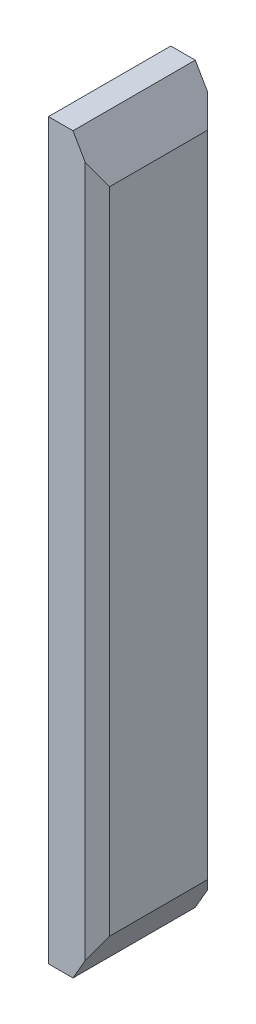
SolidWorks part; units mm, degrees
ref_plane "前视基准面" through (0, 0, 0) normal (0, 0, 1) x (1, 0, 0)
ref_plane "上视基准面" through (0, 0, 0) normal (0, 1, 0) x (1, 0, 0)
ref_plane "右视基准面" through (0, 0, 0) normal (1, 0, 0) x (0, 0, -1)
sketch "草图1" plane through (0, 0, 0) normal (1, 0, 0) x (0, 0, -1)
  line L1 (5, -30) -> (-5, -30)
  line L2 (5, -30) -> (5, 30)
  line L3 (5, 30) -> (-5, 30)
  line L4 (-5, -30) -> (-5, 30)
  line L5 (5, -30) -> (-5, 30) construction
  line L6 (5, 30) -> (-5, -30) construction
  point P0 (0, 0)
  dimension "D1" = 10
  dimension "D2" = 60
extrude "凸台-拉伸1" add sketch "草图1" along normal blind 4
chamfer "倒角1" distance 2 angle 60 4 edges at (4, 0, -5) (4, 0, 5) (4, 30, 0) (4, -30, 0)
chamfer "倒角2" distance 1 angle 45 2 edges at (4, 0, -5) (4, 0, 5)
